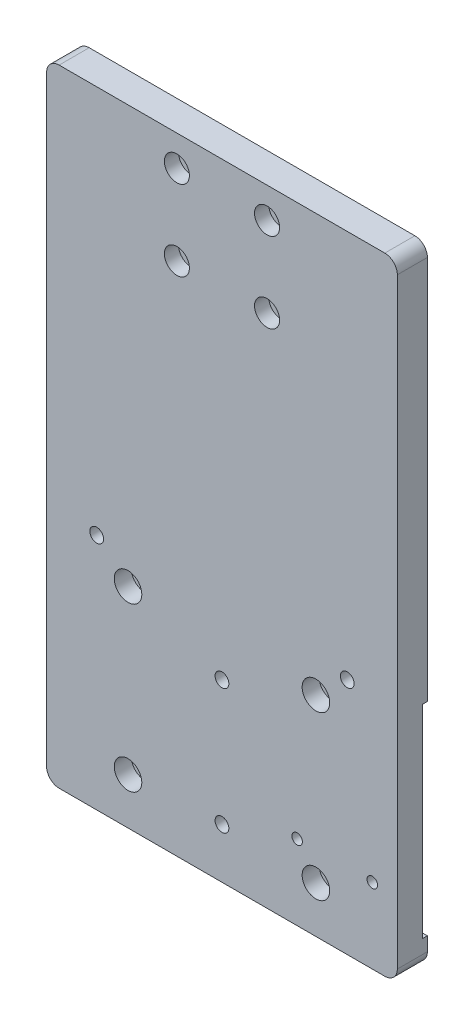
from build123d import *

# Parameters (mm, degrees)
SKETCH_1_W                = 140
SKETCH_1_H                = 250
EXTRUDE_1_DEPTH           = 12
HOLE_WIZARD_1_D           = 5.5
HOLE_WIZARD_1_DEPTH       = 15
HOLE_WIZARD_1_CBORE_D     = 10
HOLE_WIZARD_1_CBORE_DEPTH = 5.7
HOLE_WIZARD_1_TIP         = 1.652366702
HOLE_WIZARD_2_D           = 6.6
HOLE_WIZARD_2_DEPTH       = 15
HOLE_WIZARD_2_CBORE_D     = 11
HOLE_WIZARD_2_CBORE_DEPTH = 6.8
HOLE_WIZARD_2_TIP         = 1.982840043
HOLE_WIZARD_3_D           = 5.5
HOLE_WIZARD_3_DEPTH       = 14.4
HOLE_WIZARD_3_CBORE_D     = 10
HOLE_WIZARD_3_CBORE_DEPTH = 5.7
HOLE_WIZARD_3_TIP         = 1.652366702
SKETCH_8_W                = 140
SKETCH_8_H                = 81
CUT_EXTRUDE_1_DEPTH       = 2
HOLE_WIZARD_0_D           = 5.5
HOLE_WIZARD_0_CBORE_D     = 10
HOLE_WIZARD_0_CBORE_DEPTH = 7
HOLE_WIZARD_M5_1_D        = 4.2
FILLET_1_R                = 5


with BuildPart() as part:
    # 草图1 → 凸台-拉伸1 (new body)
    with BuildSketch(Plane.XY):
        Rectangle(SKETCH_1_W, SKETCH_1_H)
    extrude(amount=EXTRUDE_1_DEPTH)

    # 打孔尺寸(%根据)内六角圆柱头螺钉的类型1
    with Locations(Plane.XY.offset(12)):
        with Locations((-18, 112.800000705), (-18, 80.800000705), (18, 80.800000705), (18, 112.800000705)):
            CounterBoreHole(HOLE_WIZARD_1_D / 2, HOLE_WIZARD_1_CBORE_D / 2, HOLE_WIZARD_1_CBORE_DEPTH, depth=HOLE_WIZARD_1_DEPTH)
            with Locations((0, 0, -(HOLE_WIZARD_1_DEPTH + HOLE_WIZARD_1_TIP / 2))):  # 118° drill point
                Cone(0, HOLE_WIZARD_1_D / 2, HOLE_WIZARD_1_TIP, mode=Mode.SUBTRACT)

    # 打孔尺寸(%根据)内六角圆柱头螺钉的类型2
    with Locations(Plane.XY.offset(12)):
        with Locations((37.5, -106.499999647), (-37.5, -106.499999647), (-37.5, -41.499999647), (37.5, -41.499999647)):
            CounterBoreHole(HOLE_WIZARD_2_D / 2, HOLE_WIZARD_2_CBORE_D / 2, HOLE_WIZARD_2_CBORE_DEPTH, depth=HOLE_WIZARD_2_DEPTH)
            with Locations((0, 0, -(HOLE_WIZARD_2_DEPTH + HOLE_WIZARD_2_TIP / 2))):  # 118° drill point
                Cone(0, HOLE_WIZARD_2_D / 2, HOLE_WIZARD_2_TIP, mode=Mode.SUBTRACT)

    # 打孔尺寸(%根据)内六角圆柱头螺钉的类型3
    with Locations(Plane(origin=(0, 0, 0), x_dir=(-1, 0, 0), z_dir=(0, 0, -1))):
        with Locations((0, -105), (0, -55)):
            CounterBoreHole(HOLE_WIZARD_3_D / 2, HOLE_WIZARD_3_CBORE_D / 2, HOLE_WIZARD_3_CBORE_DEPTH, depth=HOLE_WIZARD_3_DEPTH)
            with Locations((0, 0, -(HOLE_WIZARD_3_DEPTH + HOLE_WIZARD_3_TIP / 2))):  # 118° drill point
                Cone(0, HOLE_WIZARD_3_D / 2, HOLE_WIZARD_3_TIP, mode=Mode.SUBTRACT)

    # 草图8 → 切除-拉伸1 (cut)
    with BuildSketch(Plane(origin=(0, 0, 0), x_dir=(-1, 0, 0), z_dir=(0, 0, -1))):
        with Locations((0, -73.999999647)):
            Rectangle(SKETCH_8_W, SKETCH_8_H)
    extrude(amount=-CUT_EXTRUDE_1_DEPTH, mode=Mode.SUBTRACT)

    # 打孔尺寸(%根据)内六角圆柱头螺钉的类型0 (through all)
    with Locations(Plane(origin=(0, 0, 0), x_dir=(-1, 0, 0), z_dir=(0, 0, -1))):
        with Locations((-50, -30), (50, -30)):
            CounterBoreHole(HOLE_WIZARD_0_D / 2, HOLE_WIZARD_0_CBORE_D / 2, HOLE_WIZARD_0_CBORE_DEPTH)

    # M5 螺纹孔1 (through all)
    with Locations(Plane.XY.offset(12)):
        with Locations((30, -95), (60, -95)):
            Hole(HOLE_WIZARD_M5_1_D / 2)

    # 圆角1
    fillet_1_edges = [part.edges().sort_by_distance(p)[0] for p in [
        (-70, 125, 6),
        (70, 125, 6),
        (70, -125, 6),
        (-70, -125, 6),
    ]]
    fillet(fillet_1_edges, radius=FILLET_1_R)


solid = part.part
